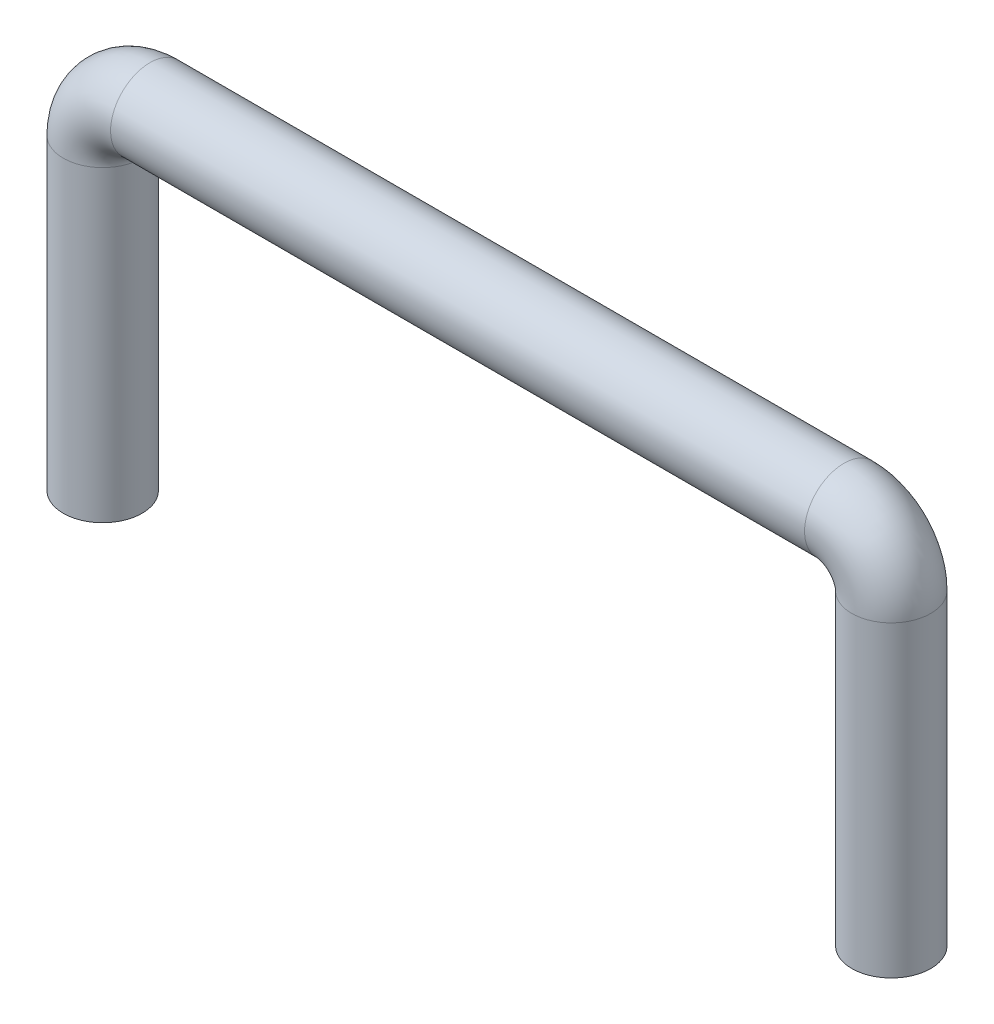
SolidWorks part; units mm, degrees
ref_plane "Front Plane" through (0, 0, 0) normal (0, 0, 1) x (1, 0, 0)
ref_plane "Top Plane" through (0, 0, 0) normal (0, 1, 0) x (1, 0, 0)
ref_plane "Right Plane" through (0, 0, 0) normal (1, 0, 0) x (0, 0, -1)
sketch "Sketch1" plane through (0, 0, 0) normal (0, 0, 1) x (1, 0, 0)
  line L0 (-15.9977, -10.4423) -> (-15.9977, 28.5577)
  line L1 (-9.9977, 34.5577) -> (78.0023, 34.5577)
  line L2 (84.0023, 28.5577) -> (84.0023, -10.4423)
  arc A0 (84.0023, 28.5577) -> (78.0023, 34.5577) centre (78.0023, 28.5577) ccw
  arc A1 (-9.9977, 34.5577) -> (-15.9977, 28.5577) centre (-9.9977, 28.5577) ccw
  point P6 (84.0023, 34.5577)
  point P9 (-15.9977, 34.5577)
  dimension "D4" = 6
  dimension "D1" = 45
  dimension "D2" = 45
  dimension "D3" = 100
ref_plane "Plane1" through (-15.9977, -10.4423, 0) normal (0, 1, 0) x (-1, 0, 0)
sketch "Sketch2" plane through (-15.9977, -10.4423, 0) normal (0, 1, 0) x (-1, 0, 0)
  circle A0 centre (0, 0) radius 5
sweep "Sweep1" add profiles "Sketch2" path "Sketch1"
